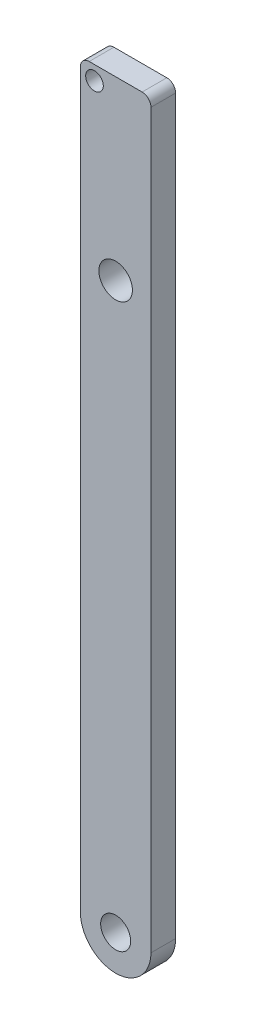
from build123d import *

# Parameters (mm, degrees)
SKETCH_1_R          = 9.5
SKETCH_1_R_2        = 8.5
EXTRUDE_1_DEPTH     = 14
SKETCH_2_R          = 5
CUT_EXTRUDE_1_DEPTH = 20


with BuildPart() as part:
    # 草图1 → 凸台-拉伸1 (new body)
    with BuildSketch(Plane.XY):
        with BuildLine():
            Line((-15, 220), (15, 220))
            ThreePointArc((15, 220), (18.535533906, 218.535533906), (20, 215))
            Line((20, 215), (20, -200))
            ThreePointArc((20, -200), (0, -220), (-20, -200))
            Line((-20, -200), (-20, 215))
            ThreePointArc((-20, 215), (-18.535533906, 218.535533906), (-15, 220))
        make_face()
        with Locations((0, 120)):
            Circle(SKETCH_1_R, mode=Mode.SUBTRACT)
        with Locations((0, -200)):
            Circle(SKETCH_1_R_2, mode=Mode.SUBTRACT)
    extrude(amount=EXTRUDE_1_DEPTH)

    # 草图2 → 切除-拉伸1 (cut)
    with BuildSketch(Plane(origin=(0, 0, 0), x_dir=(-1, 0, 0), z_dir=(0, 0, -1))):
        with Locations((12, 212)):
            Circle(SKETCH_2_R)
    extrude(amount=-CUT_EXTRUDE_1_DEPTH, mode=Mode.SUBTRACT)


solid = part.part
